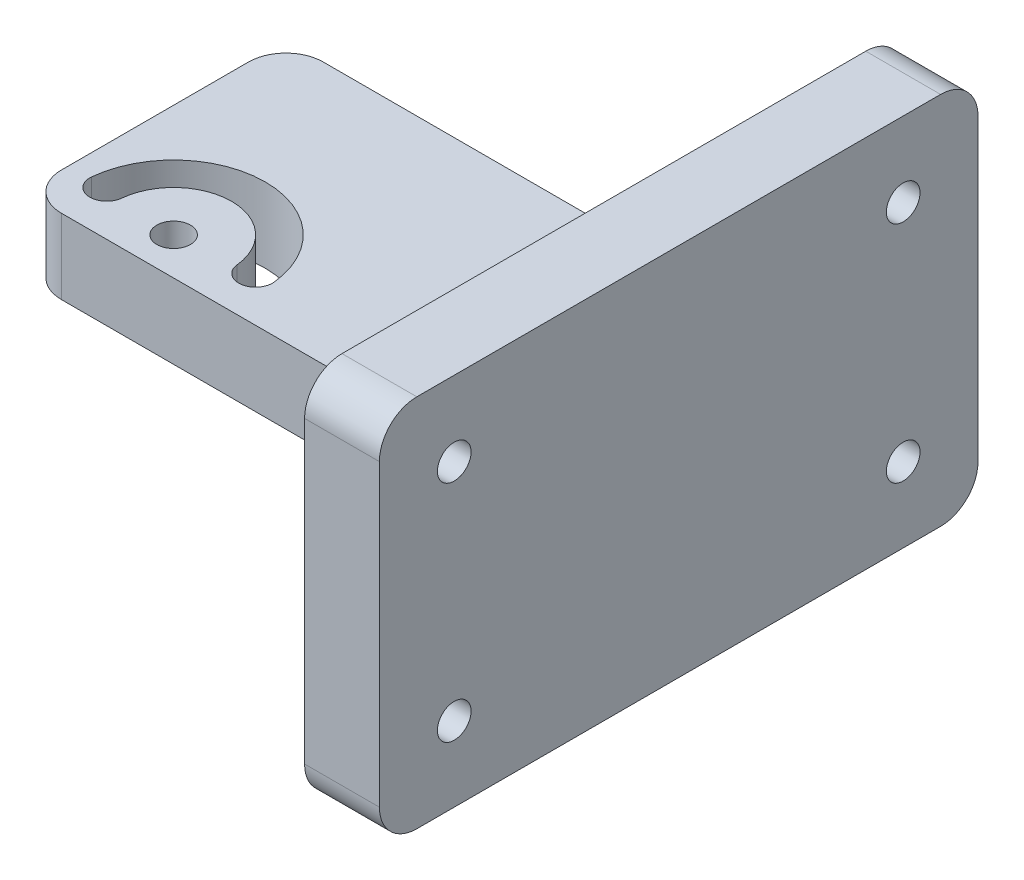
from build123d import *

# Parameters (mm, degrees)
SKETCH_1_W                   = 60
SKETCH_1_H                   = 35
EXTRUDE_1_DEPTH              = 5
SKETCH_2_R                   = 2.25
CUT_EXTRUDE_1_DEPTH          = 37.142080737
CUT_EXTRUDE_2_DEPTH          = 37.142080737
SKETCH_5_W                   = 80
SKETCH_5_H                   = 50
EXTRUDE_3_DEPTH              = 10
HOLE_WIZARD_M4_1_D           = 4.5
HOLE_WIZARD_M4_1_CBORE_D     = 8
HOLE_WIZARD_M4_1_CBORE_DEPTH = 4.4
FILLET_1_R                   = 5


with BuildPart() as part:
    # 草图1 → 凸台-拉伸1 (new, symmetric)
    with BuildSketch(Plane(origin=(0, 0, 0), x_dir=(1, 0, 0), z_dir=(0, 1, 0))):
        Rectangle(SKETCH_1_W, SKETCH_1_H)
    extrude(amount=EXTRUDE_1_DEPTH, both=True)

    # 草图2 → 切除-拉伸1 (cut, through all)
    with BuildSketch(Plane.XZ.offset(5)):
        with Locations(Location((-15, 12.5, 0), (0, 0, 270))):
            Circle(SKETCH_2_R)
        with Locations(Location((-15, 2.5, 0), (0, 0, 270))):
            Circle(SKETCH_2_R)
    extrude(amount=-CUT_EXTRUDE_1_DEPTH, mode=Mode.SUBTRACT)

    # 草图3 → 切除-拉伸2 (cut, through all)
    with BuildSketch(Plane.XZ.offset(5)):
        with BuildLine():
            ThreePointArc((-27.188596105, 11.275), (-15, 0.25), (-2.811403895, 11.275))
            ThreePointArc((-2.811403895, 11.275), (-4.825125629, 13.738721733), (-7.288847362, 11.725))
            ThreePointArc((-7.288847362, 11.725), (-15, 4.75), (-22.711152638, 11.725))
            ThreePointArc((-22.711152638, 11.725), (-25.174874371, 13.738721733), (-27.188596105, 11.275))
        make_face()
    extrude(amount=-CUT_EXTRUDE_2_DEPTH, mode=Mode.SUBTRACT)

    # 草图5 → 凸台-拉伸3 (add)
    with BuildSketch(Plane(origin=(30, 0, 0), x_dir=(0, 0, -1), z_dir=(1, 0, 0))):
        Rectangle(SKETCH_5_W, SKETCH_5_H)
    extrude(amount=EXTRUDE_3_DEPTH)

    # M4 六角凹头螺钉的柱形沉头孔1 (through all)
    with Locations(Plane.ZY.offset(-30)):
        with Locations((30, 15), (-30, 15), (-30, -15), (30, -15)):
            CounterBoreHole(HOLE_WIZARD_M4_1_D / 2, HOLE_WIZARD_M4_1_CBORE_D / 2, HOLE_WIZARD_M4_1_CBORE_DEPTH)

    # 圆角1
    fillet_1_edges = [part.edges().sort_by_distance(p)[0] for p in [
        (35, -25, -40),
        (35, 25, -40),
        (35, 25, 40),
        (35, -25, 40),
        (-30, 0, 17.5),
        (-30, 0, -17.5),
    ]]
    fillet(fillet_1_edges, radius=FILLET_1_R)


solid = part.part
